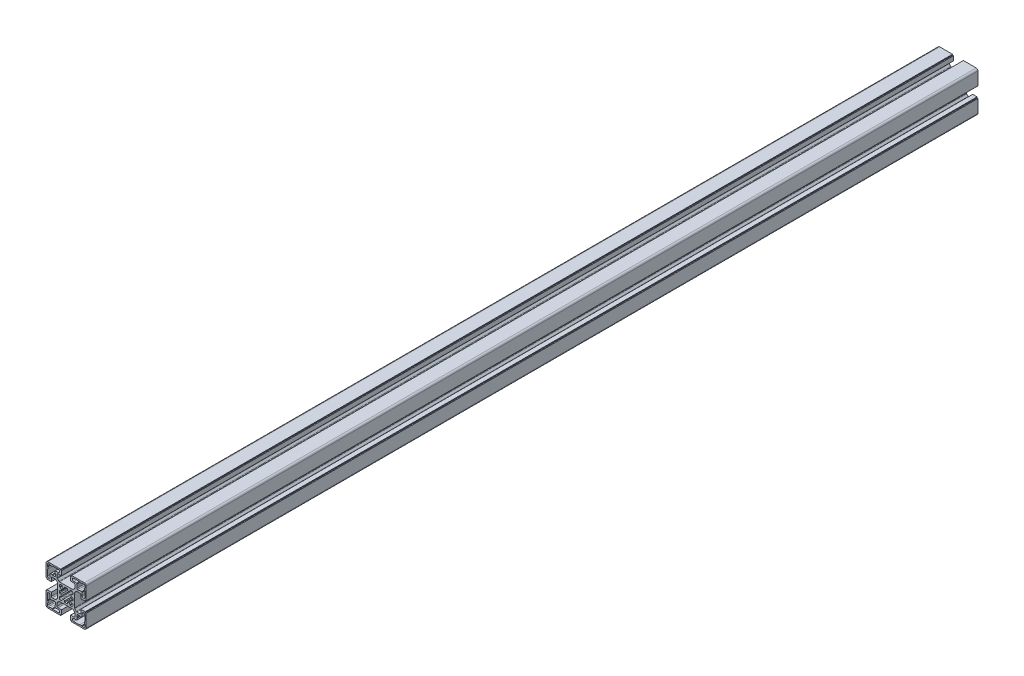
SolidWorks part; units mm, degrees
material "1.11.45.045045.04"
ref_plane "前视基准面" through (0, 0, 0) normal (0, 0, 1) x (1, 0, 0)
ref_plane "上视基准面" through (0, 0, 0) normal (0, 1, 0) x (1, 0, 0)
ref_plane "右视基准面" through (0, 0, 0) normal (1, 0, 0) x (0, 0, -1)
sketch "草图1" plane through (0, 0, 0) normal (0, 0, 1) x (1, 0, 0)
  line L0 (30.535, 44.0271) -> (29.0823, 45.4798)
  line L1 (31.4137, 44.0271) -> (30.535, 44.0271)
  line L2 (31.4137, 42.0271) -> (31.4137, 44.0271)
  line L3 (28.4137, 41.0271) -> (30.4137, 41.0271)
  line L4 (28.4137, 41.9058) -> (28.4137, 41.0271)
  line L5 (26.961, 43.3585) -> (28.4137, 41.9058)
  line L6 (25.4137, 41.0271) -> (25.4137, 42.7176)
  line L7 (22.4137, 41.0271) -> (25.4137, 41.0271)
  line L8 (22.4137, 42.7176) -> (22.4137, 41.0271)
  line L9 (19.4137, 41.9058) -> (20.8664, 43.3585)
  line L10 (19.4137, 41.0271) -> (19.4137, 41.9058)
  line L11 (17.4137, 41.0271) -> (19.4137, 41.0271)
  line L12 (16.4137, 44.0271) -> (16.4137, 42.0271)
  line L13 (17.2924, 44.0271) -> (16.4137, 44.0271)
  line L14 (18.7451, 45.4798) -> (17.2924, 44.0271)
  line L15 (16.4137, 47.0271) -> (18.1042, 47.0271)
  line L16 (16.4137, 50.0271) -> (16.4137, 47.0271)
  line L17 (18.1042, 50.0271) -> (16.4137, 50.0271)
  line L18 (17.2924, 53.0271) -> (18.7451, 51.5744)
  line L19 (16.4137, 53.0271) -> (17.2924, 53.0271)
  line L20 (16.4137, 55.0271) -> (16.4137, 53.0271)
  line L21 (19.4137, 56.0271) -> (17.4137, 56.0271)
  line L22 (19.4137, 55.1484) -> (19.4137, 56.0271)
  line L23 (20.8664, 53.6957) -> (19.4137, 55.1484)
  line L24 (22.4137, 56.0271) -> (22.4137, 54.3366)
  line L25 (25.4137, 56.0271) -> (22.4137, 56.0271)
  line L26 (25.4137, 54.3366) -> (25.4137, 56.0271)
  line L27 (28.4137, 55.1484) -> (26.961, 53.6957)
  line L28 (28.4137, 56.0271) -> (28.4137, 55.1484)
  line L29 (30.4137, 56.0271) -> (28.4137, 56.0271)
  line L30 (31.4137, 53.0271) -> (31.4137, 55.0271)
  line L31 (30.535, 53.0271) -> (31.4137, 53.0271)
  line L32 (29.0823, 51.5744) -> (30.535, 53.0271)
  line L33 (31.4137, 50.0271) -> (29.7232, 50.0271)
  line L34 (31.4137, 47.0271) -> (31.4137, 50.0271)
  line L35 (29.7232, 47.0271) -> (31.4137, 47.0271)
  line L36 (11.4137, 66.0271) -> (11.9137, 66.5271)
  line L37 (11.4137, 64.0271) -> (11.4137, 66.0271)
  line L38 (11.9137, 63.5271) -> (11.4137, 64.0271)
  line L39 (11.9137, 61.5271) -> (11.9137, 63.5271)
  line L40 (8.9137, 60.5271) -> (10.9137, 60.5271)
  line L41 (8.4137, 61.0271) -> (8.9137, 60.5271)
  line L42 (6.4137, 61.0271) -> (8.4137, 61.0271)
  line L43 (5.9137, 60.5271) -> (6.4137, 61.0271)
  line L44 (5.9137, 57.1271) -> (5.9137, 60.5271)
  line L45 (2.9137, 63.5271) -> (2.9137, 57.1271)
  line L46 (3.4137, 64.0271) -> (2.9137, 63.5271)
  line L47 (3.4137, 66.0271) -> (3.4137, 64.0271)
  line L48 (2.9137, 66.5271) -> (3.4137, 66.0271)
  line L49 (2.9137, 68.5271) -> (2.9137, 66.5271)
  line L50 (5.9137, 69.5271) -> (3.9137, 69.5271)
  line L51 (6.4137, 69.0271) -> (5.9137, 69.5271)
  line L52 (8.4137, 69.0271) -> (6.4137, 69.0271)
  line L53 (8.9137, 69.5271) -> (8.4137, 69.0271)
  line L54 (15.3137, 69.5271) -> (8.9137, 69.5271)
  line L55 (11.9137, 66.5271) -> (15.3137, 66.5271)
  line L56 (11.9137, 30.5271) -> (11.4137, 31.0271)
  line L57 (15.3137, 30.5271) -> (11.9137, 30.5271)
  line L58 (8.9137, 27.5271) -> (15.3137, 27.5271)
  line L59 (8.4137, 28.0271) -> (8.9137, 27.5271)
  line L60 (6.4137, 28.0271) -> (8.4137, 28.0271)
  line L61 (5.9137, 27.5271) -> (6.4137, 28.0271)
  line L62 (3.9137, 27.5271) -> (5.9137, 27.5271)
  line L63 (2.9137, 30.5271) -> (2.9137, 28.5271)
  line L64 (3.4137, 31.0271) -> (2.9137, 30.5271)
  line L65 (3.4137, 33.0271) -> (3.4137, 31.0271)
  line L66 (2.9137, 33.5271) -> (3.4137, 33.0271)
  line L67 (2.9137, 39.9271) -> (2.9137, 33.5271)
  line L68 (5.9137, 36.5271) -> (5.9137, 39.9271)
  line L69 (6.4137, 36.0271) -> (5.9137, 36.5271)
  line L70 (8.4137, 36.0271) -> (6.4137, 36.0271)
  line L71 (8.9137, 36.5271) -> (8.4137, 36.0271)
  line L72 (10.9137, 36.5271) -> (8.9137, 36.5271)
  line L73 (11.9137, 33.5271) -> (11.9137, 35.5271)
  line L74 (11.4137, 33.0271) -> (11.9137, 33.5271)
  line L75 (11.4137, 31.0271) -> (11.4137, 33.0271)
  line L76 (41.9137, 36.5271) -> (41.4137, 36.0271)
  line L77 (41.9137, 39.9271) -> (41.9137, 36.5271)
  line L78 (44.9137, 33.5271) -> (44.9137, 39.9271)
  line L79 (44.4137, 33.0271) -> (44.9137, 33.5271)
  line L80 (44.4137, 31.0271) -> (44.4137, 33.0271)
  line L81 (44.9137, 30.5271) -> (44.4137, 31.0271)
  line L82 (44.9137, 28.5271) -> (44.9137, 30.5271)
  line L83 (41.9137, 27.5271) -> (43.9137, 27.5271)
  line L84 (41.4137, 28.0271) -> (41.9137, 27.5271)
  line L85 (39.4137, 28.0271) -> (41.4137, 28.0271)
  line L86 (38.9137, 27.5271) -> (39.4137, 28.0271)
  line L87 (32.5137, 27.5271) -> (38.9137, 27.5271)
  line L88 (35.9137, 30.5271) -> (32.5137, 30.5271)
  line L89 (36.4137, 31.0271) -> (35.9137, 30.5271)
  line L90 (36.4137, 33.0271) -> (36.4137, 31.0271)
  line L91 (35.9137, 33.5271) -> (36.4137, 33.0271)
  line L92 (35.9137, 35.5271) -> (35.9137, 33.5271)
  line L93 (38.9137, 36.5271) -> (36.9137, 36.5271)
  line L94 (39.4137, 36.0271) -> (38.9137, 36.5271)
  line L95 (41.4137, 36.0271) -> (39.4137, 36.0271)
  line L96 (35.9137, 66.5271) -> (36.4137, 66.0271)
  line L97 (32.5137, 66.5271) -> (35.9137, 66.5271)
  line L98 (38.9137, 69.5271) -> (32.5137, 69.5271)
  line L99 (39.4137, 69.0271) -> (38.9137, 69.5271)
  line L100 (41.4137, 69.0271) -> (39.4137, 69.0271)
  line L101 (41.9137, 69.5271) -> (41.4137, 69.0271)
  line L102 (43.9137, 69.5271) -> (41.9137, 69.5271)
  line L103 (44.9137, 66.5271) -> (44.9137, 68.5271)
  line L104 (44.4137, 66.0271) -> (44.9137, 66.5271)
  line L105 (44.4137, 64.0271) -> (44.4137, 66.0271)
  line L106 (44.9137, 63.5271) -> (44.4137, 64.0271)
  line L107 (44.9137, 57.1271) -> (44.9137, 63.5271)
  line L108 (41.9137, 60.5271) -> (41.9137, 57.1271)
  line L109 (41.4137, 61.0271) -> (41.9137, 60.5271)
  line L110 (39.4137, 61.0271) -> (41.4137, 61.0271)
  line L111 (38.9137, 60.5271) -> (39.4137, 61.0271)
  line L112 (36.9137, 60.5271) -> (38.9137, 60.5271)
  line L113 (35.9137, 63.5271) -> (35.9137, 61.5271)
  line L114 (36.4137, 64.0271) -> (35.9137, 63.5271)
  line L115 (36.4137, 66.0271) -> (36.4137, 64.0271)
  line L116 (33.7066, 40.502) -> (35.3886, 38.82)
  line L117 (33.4137, 55.8451) -> (33.4137, 41.2091)
  line L118 (35.3886, 58.2342) -> (33.7066, 56.5522)
  line L119 (39.4137, 58.5271) -> (36.0957, 58.5271)
  line L120 (40.4137, 53.6271) -> (40.4137, 57.5271)
  line L121 (45.4137, 53.6271) -> (40.4137, 53.6271)
  line L122 (45.4137, 54.6271) -> (45.4137, 53.6271)
  line L123 (46.4137, 54.6271) -> (45.4137, 54.6271)
  line L124 (46.4137, 69.0271) -> (46.4137, 54.6271)
  line L125 (30.0137, 71.0271) -> (44.4137, 71.0271)
  line L126 (30.0137, 70.0271) -> (30.0137, 71.0271)
  line L127 (29.0137, 70.0271) -> (30.0137, 70.0271)
  line L128 (29.0137, 65.0271) -> (29.0137, 70.0271)
  line L129 (32.9137, 65.0271) -> (29.0137, 65.0271)
  line L130 (33.9137, 60.7091) -> (33.9137, 64.0271)
  line L131 (31.9388, 58.32) -> (33.6208, 60.002)
  line L132 (16.5957, 58.0271) -> (31.2317, 58.0271)
  line L133 (14.2066, 60.002) -> (15.8886, 58.32)
  line L134 (13.9137, 64.0271) -> (13.9137, 60.7091)
  line L135 (18.8137, 65.0271) -> (14.9137, 65.0271)
  line L136 (18.8137, 70.0271) -> (18.8137, 65.0271)
  line L137 (17.8137, 70.0271) -> (18.8137, 70.0271)
  line L138 (17.8137, 71.0271) -> (17.8137, 70.0271)
  line L139 (3.4137, 71.0271) -> (17.8137, 71.0271)
  line L140 (1.4137, 54.6271) -> (1.4137, 69.0271)
  line L141 (2.4137, 54.6271) -> (1.4137, 54.6271)
  line L142 (2.4137, 53.6271) -> (2.4137, 54.6271)
  line L143 (7.4137, 53.6271) -> (2.4137, 53.6271)
  line L144 (7.4137, 57.5271) -> (7.4137, 53.6271)
  line L145 (11.7317, 58.5271) -> (8.4137, 58.5271)
  line L146 (14.1208, 56.5522) -> (12.4388, 58.2342)
  line L147 (14.4137, 41.2091) -> (14.4137, 55.8451)
  line L148 (12.4388, 38.82) -> (14.1208, 40.502)
  line L149 (8.4137, 38.5271) -> (11.7317, 38.5271)
  line L150 (7.4137, 43.4271) -> (7.4137, 39.5271)
  line L151 (2.4137, 43.4271) -> (7.4137, 43.4271)
  line L152 (2.4137, 42.4271) -> (2.4137, 43.4271)
  line L153 (1.4137, 42.4271) -> (2.4137, 42.4271)
  line L154 (1.4137, 28.0271) -> (1.4137, 42.4271)
  line L155 (17.8137, 26.0271) -> (3.4137, 26.0271)
  line L156 (17.8137, 27.0271) -> (17.8137, 26.0271)
  line L157 (18.8137, 27.0271) -> (17.8137, 27.0271)
  line L158 (18.8137, 32.0271) -> (18.8137, 27.0271)
  line L159 (14.9137, 32.0271) -> (18.8137, 32.0271)
  line L160 (13.9137, 36.3451) -> (13.9137, 33.0271)
  line L161 (15.8886, 38.7342) -> (14.2066, 37.0522)
  line L162 (31.2317, 39.0271) -> (16.5957, 39.0271)
  line L163 (33.6208, 37.0522) -> (31.9388, 38.7342)
  line L164 (33.9137, 33.0271) -> (33.9137, 36.3451)
  line L165 (29.0137, 32.0271) -> (32.9137, 32.0271)
  line L166 (29.0137, 27.0271) -> (29.0137, 32.0271)
  line L167 (30.0137, 27.0271) -> (29.0137, 27.0271)
  line L168 (30.0137, 26.0271) -> (30.0137, 27.0271)
  line L169 (44.4137, 26.0271) -> (30.0137, 26.0271)
  line L170 (46.4137, 42.4271) -> (46.4137, 28.0271)
  line L171 (45.4137, 42.4271) -> (46.4137, 42.4271)
  line L172 (45.4137, 43.4271) -> (45.4137, 42.4271)
  line L173 (40.4137, 43.4271) -> (45.4137, 43.4271)
  line L174 (40.4137, 39.5271) -> (40.4137, 43.4271)
  line L175 (36.0957, 38.5271) -> (39.4137, 38.5271)
  arc A0 (30.4137, 41.0271) -> (31.4137, 42.0271) centre (30.4137, 42.0271) ccw
  arc A1 (25.4137, 42.7176) -> (26.961, 43.3585) centre (23.9137, 48.5271) ccw
  arc A2 (20.8664, 43.3585) -> (22.4137, 42.7176) centre (23.9137, 48.5271) ccw
  arc A3 (16.4137, 42.0271) -> (17.4137, 41.0271) centre (17.4137, 42.0271) ccw
  arc A4 (18.1042, 47.0271) -> (18.7451, 45.4798) centre (23.9137, 48.5271) ccw
  arc A5 (18.7451, 51.5744) -> (18.1042, 50.0271) centre (23.9137, 48.5271) ccw
  arc A6 (17.4137, 56.0271) -> (16.4137, 55.0271) centre (17.4137, 55.0271) ccw
  arc A7 (22.4137, 54.3366) -> (20.8664, 53.6957) centre (23.9137, 48.5271) ccw
  arc A8 (26.961, 53.6957) -> (25.4137, 54.3366) centre (23.9137, 48.5271) ccw
  arc A9 (31.4137, 55.0271) -> (30.4137, 56.0271) centre (30.4137, 55.0271) ccw
  arc A10 (29.7232, 50.0271) -> (29.0823, 51.5744) centre (23.9137, 48.5271) ccw
  arc A11 (29.0823, 45.4798) -> (29.7232, 47.0271) centre (23.9137, 48.5271) ccw
  arc A12 (10.9137, 60.5271) -> (11.9137, 61.5271) centre (10.9137, 61.5271) ccw
  arc A13 (2.9137, 57.1271) -> (5.9137, 57.1271) centre (4.4137, 57.1271) ccw
  arc A14 (3.9137, 69.5271) -> (2.9137, 68.5271) centre (3.9137, 68.5271) ccw
  arc A15 (15.3137, 66.5271) -> (15.3137, 69.5271) centre (15.3137, 68.0271) ccw
  arc A16 (15.3137, 27.5271) -> (15.3137, 30.5271) centre (15.3137, 29.0271) ccw
  arc A17 (2.9137, 28.5271) -> (3.9137, 27.5271) centre (3.9137, 28.5271) ccw
  arc A18 (5.9137, 39.9271) -> (2.9137, 39.9271) centre (4.4137, 39.9271) ccw
  arc A19 (11.9137, 35.5271) -> (10.9137, 36.5271) centre (10.9137, 35.5271) ccw
  arc A20 (44.9137, 39.9271) -> (41.9137, 39.9271) centre (43.4137, 39.9271) ccw
  arc A21 (43.9137, 27.5271) -> (44.9137, 28.5271) centre (43.9137, 28.5271) ccw
  arc A22 (32.5137, 30.5271) -> (32.5137, 27.5271) centre (32.5137, 29.0271) ccw
  arc A23 (36.9137, 36.5271) -> (35.9137, 35.5271) centre (36.9137, 35.5271) ccw
  arc A24 (32.5137, 69.5271) -> (32.5137, 66.5271) centre (32.5137, 68.0271) ccw
  arc A25 (44.9137, 68.5271) -> (43.9137, 69.5271) centre (43.9137, 68.5271) ccw
  arc A26 (41.9137, 57.1271) -> (44.9137, 57.1271) centre (43.4137, 57.1271) ccw
  arc A27 (35.9137, 61.5271) -> (36.9137, 60.5271) centre (36.9137, 61.5271) ccw
  arc A28 (35.3886, 38.82) -> (36.0957, 38.5271) centre (36.0957, 39.5271) ccw
  arc A29 (33.4137, 41.2091) -> (33.7066, 40.502) centre (34.4137, 41.2091) ccw
  arc A30 (33.7066, 56.5522) -> (33.4137, 55.8451) centre (34.4137, 55.8451) ccw
  arc A31 (36.0957, 58.5271) -> (35.3886, 58.2342) centre (36.0957, 57.5271) ccw
  arc A32 (40.4137, 57.5271) -> (39.4137, 58.5271) centre (39.4137, 57.5271) ccw
  arc A33 (46.4137, 69.0271) -> (44.4137, 71.0271) centre (44.4137, 69.0271) ccw
  arc A34 (33.9137, 64.0271) -> (32.9137, 65.0271) centre (32.9137, 64.0271) ccw
  arc A35 (33.6208, 60.002) -> (33.9137, 60.7091) centre (32.9137, 60.7091) ccw
  arc A36 (31.2317, 58.0271) -> (31.9388, 58.32) centre (31.2317, 59.0271) ccw
  arc A37 (15.8886, 58.32) -> (16.5957, 58.0271) centre (16.5957, 59.0271) ccw
  arc A38 (13.9137, 60.7091) -> (14.2066, 60.002) centre (14.9137, 60.7091) ccw
  arc A39 (14.9137, 65.0271) -> (13.9137, 64.0271) centre (14.9137, 64.0271) ccw
  arc A40 (3.4137, 71.0271) -> (1.4137, 69.0271) centre (3.4137, 69.0271) ccw
  arc A41 (8.4137, 58.5271) -> (7.4137, 57.5271) centre (8.4137, 57.5271) ccw
  arc A42 (12.4388, 58.2342) -> (11.7317, 58.5271) centre (11.7317, 57.5271) ccw
  arc A43 (14.4137, 55.8451) -> (14.1208, 56.5522) centre (13.4137, 55.8451) ccw
  arc A44 (14.1208, 40.502) -> (14.4137, 41.2091) centre (13.4137, 41.2091) ccw
  arc A45 (11.7317, 38.5271) -> (12.4388, 38.82) centre (11.7317, 39.5271) ccw
  arc A46 (7.4137, 39.5271) -> (8.4137, 38.5271) centre (8.4137, 39.5271) ccw
  arc A47 (1.4137, 28.0271) -> (3.4137, 26.0271) centre (3.4137, 28.0271) ccw
  arc A48 (13.9137, 33.0271) -> (14.9137, 32.0271) centre (14.9137, 33.0271) ccw
  arc A49 (14.2066, 37.0522) -> (13.9137, 36.3451) centre (14.9137, 36.3451) ccw
  arc A50 (16.5957, 39.0271) -> (15.8886, 38.7342) centre (16.5957, 38.0271) ccw
  arc A51 (31.9388, 38.7342) -> (31.2317, 39.0271) centre (31.2317, 38.0271) ccw
  arc A52 (33.9137, 36.3451) -> (33.6208, 37.0522) centre (32.9137, 36.3451) ccw
  arc A53 (32.9137, 32.0271) -> (33.9137, 33.0271) centre (32.9137, 33.0271) ccw
  arc A54 (44.4137, 26.0271) -> (46.4137, 28.0271) centre (44.4137, 28.0271) ccw
  arc A55 (39.4137, 38.5271) -> (40.4137, 39.5271) centre (39.4137, 39.5271) ccw
extrude "拉伸1" add sketch "草图1" along normal blind 1000
